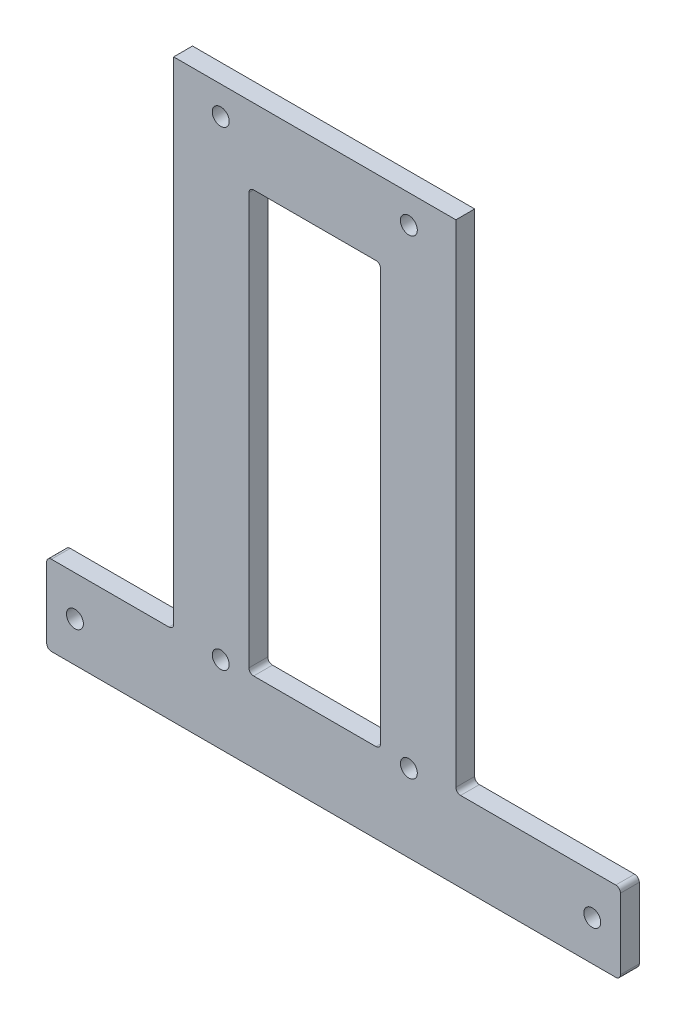
SolidWorks part; units mm, degrees
material "Q235B"
ref_plane "Front Plane" through (0, 0, 0) normal (0, 0, 1) x (1, 0, 0)
ref_plane "Top Plane" through (0, 0, 0) normal (0, 1, 0) x (1, 0, 0)
ref_plane "Right Plane" through (0, 0, 0) normal (1, 0, 0) x (0, 0, -1)
sketch "Sketch1" plane through (0, 0, 0) normal (0, 0, 1) x (1, 0, 0)
  line L0 (5, 0) -> (605, 0)
  line L1 (610, 5) -> (610, 80)
  line L2 (605, 85) -> (440, 85)
  line L3 (435, 90) -> (435, 612.5)
  line L4 (435, 612.5) -> (135, 612.5)
  line L5 (135, 612.5) -> (135, 90)
  line L6 (130, 85) -> (5, 85)
  line L7 (0, 80) -> (0, 5)
  line L9 (220, 85) -> (350, 85)
  line L10 (215, 90) -> (215, 527.5)
  line L11 (220, 532.5) -> (350, 532.5)
  line L12 (355, 90) -> (355, 527.5)
  arc A0 (610, 80) -> (605, 85) centre (605, 80) ccw
  arc A1 (605, 0) -> (610, 5) centre (605, 5) ccw
  arc A2 (5, 0) -> (0, 5) centre (5, 5) cw
  arc A3 (5, 85) -> (0, 80) centre (5, 80) ccw
  arc A4 (215, 527.5) -> (220, 532.5) centre (220, 527.5) cw
  arc A5 (350, 532.5) -> (355, 527.5) centre (350, 527.5) cw
  arc A6 (440, 85) -> (435, 90) centre (440, 90) cw
  arc A7 (350, 85) -> (355, 90) centre (350, 90) ccw
  arc A8 (220, 85) -> (215, 90) centre (220, 90) cw
  arc A9 (135, 90) -> (130, 85) centre (130, 90) cw
  circle A10 centre (30, 42.5) radius 9
  circle A11 centre (580, 42.5) radius 9
  circle A12 centre (185, 582.5) radius 9
  circle A13 centre (385, 582.5) radius 9
  circle A14 centre (185, 82.5) radius 9
  circle A15 centre (385, 82.5) radius 9
  point P17 (610, 0)
  point P20 (0, 0)
  dimension "D10" = 5
  dimension "D12" = 550
  dimension "D13" = 30
  dimension "D14" = 18
  dimension "D15" = 18
  dimension "D16" = 42.5
  dimension "D17" = 42.5
  dimension "D18" = 200
  dimension "D19" = 500
  dimension "D20" = 50
  dimension "D21" = 540
  dimension "D1" = 610
  dimension "D2" = 85
  dimension "D3" = 135
  dimension "D4" = 85
  dimension "D5" = 80
  dimension "D6" = 175
  dimension "D7" = 80
  dimension "D8" = 612.5
  dimension "D9" = 447.5
  dimension "D11" = 85
extrude "Boss-Extrude1" add sketch "Sketch1" along normal blind 20
